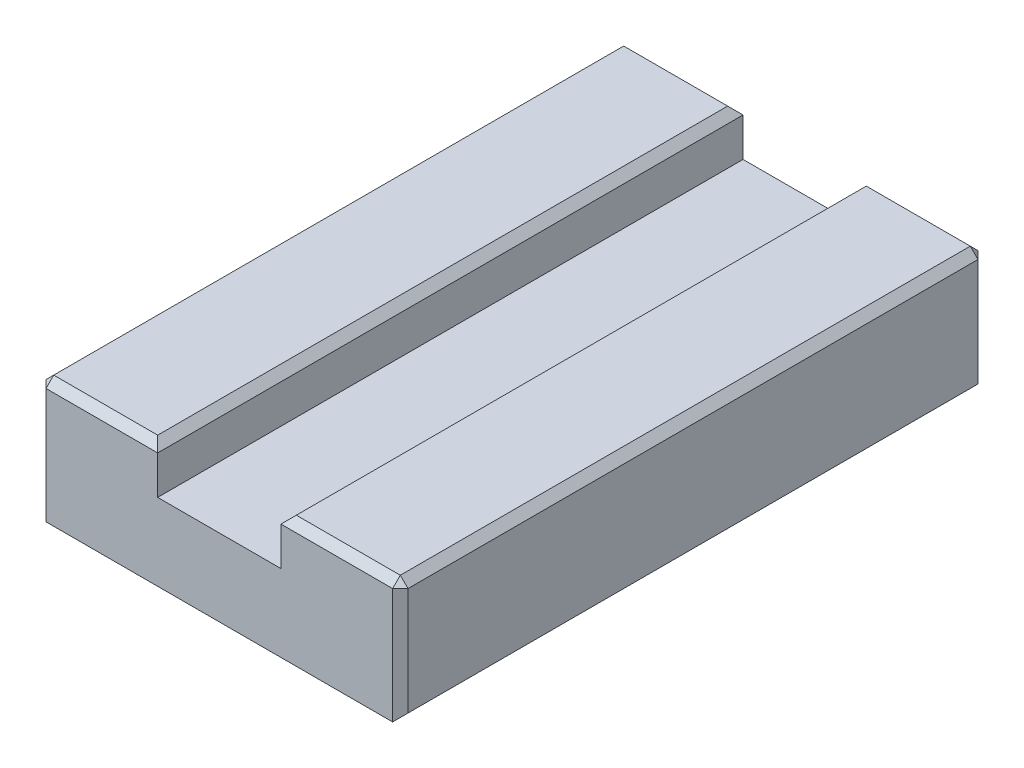
from build123d import *

# Parameters (mm, degrees)
BOSS_EXTRUDE1_DEPTH = 38
CHAMFER1_SIZE       = 0.5


with BuildPart() as part:
    # Sketch1 → Boss-Extrude1 (new body)
    with BuildSketch(Plane.XY):
        Polygon((-11.75, 4), (-4, 4), (-4, 1), (4, 1), (4, 4), (11.75, 4), (11.75, -4), (-11.75, -4), align=None)
    extrude(amount=BOSS_EXTRUDE1_DEPTH)

    # Chamfer1
    chamfer1_edges = [part.edges().sort_by_distance(p)[0] for p in [
        (7.875, 4, 0),
        (11.75, 0, 0),
        (11.75, -4, 19),
        (-11.75, -4, 19),
        (-11.75, 4, 19),
        (-4, 4, 19),
        (4, 4, 19),
        (11.75, 4, 19),
        (-7.875, 4, 38),
        (-11.75, 0, 38),
        (11.75, 0, 38),
        (7.875, 4, 38),
        (-11.75, 0, 0),
        (-7.875, 4, 0),
    ]]
    chamfer(chamfer1_edges, length=CHAMFER1_SIZE)


solid = part.part
